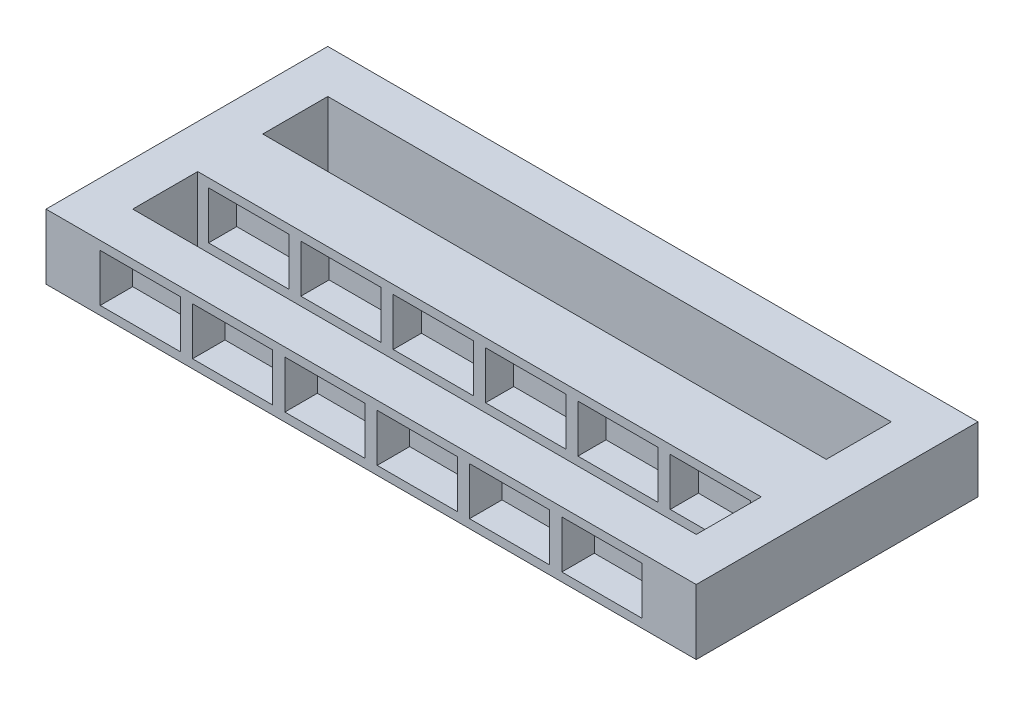
SolidWorks part; units mm, degrees
ref_plane "Front Plane" through (0, 0, 0) normal (0, 0, 1) x (1, 0, 0)
ref_plane "Top Plane" through (0, 0, 0) normal (0, 1, 0) x (1, 0, 0)
ref_plane "Right Plane" through (0, 0, 0) normal (1, 0, 0) x (0, 0, -1)
other "Configuration Table"
sketch "Sketch1" plane through (0, 0, 0) normal (0, 1, 0) x (1, 0, 0)
  line L1 (-1500, 650) -> (1500, 650)
  line L2 (-1500, 650) -> (-1500, -650)
  line L3 (-1500, -650) -> (1500, -650)
  line L4 (1500, 650) -> (1500, -650)
  line L5 (-1500, 650) -> (1500, -650) construction
  line L6 (-1500, -650) -> (1500, 650) construction
  line L7 (-1300, 450) -> (1300, 450)
  line L8 (-1300, 450) -> (-1300, 150)
  line L9 (-1300, 150) -> (1300, 150)
  line L10 (1300, 450) -> (1300, 150)
  line L11 (-1300, -150) -> (1300, -150)
  line L12 (-1300, -150) -> (-1300, -450)
  line L13 (-1300, -450) -> (1300, -450)
  line L14 (1300, -150) -> (1300, -450)
  point P0 (0, 0)
  dimension "D1" = 1300
  dimension "D2" = 3000
  dimension "D3" = 200
  dimension "D4" = 200
  dimension "D5" = 200
  dimension "D6" = 200
  dimension "D7" = 200
  dimension "D8" = 200
  dimension "D9" = 500
  dimension "D10" = 300
extrude "Boss-Extrude1" add sketch "Sketch1" along normal blind 300
sketch "Sketch2" plane through (0, 0, 650) normal (0, 0, 1) x (1, 0, 0)
  line L0 (-1500, 300) -> (-1500, 0) construction
  line L1 (-1250, 260) -> (-880, 260)
  line L2 (-1250, 260) -> (-1250, 40)
  line L3 (-1250, 40) -> (-880, 40)
  line L4 (1250, 260) -> (1250, 40)
  line L5 (1500, 300) -> (1500, 0) construction
  line L6 (-1500, 0) -> (1500, 0) construction
  line L7 (-1500, 300) -> (1500, 300) construction
  line L8 (-880, 260) -> (-880, 40)
  line L9 (-824, 260) -> (-824, 40)
  line L10 (-454, 260) -> (-454, 40)
  line L11 (-398, 260) -> (-398, 40)
  line L12 (-28, 260) -> (-28, 40)
  line L13 (28, 260) -> (28, 40)
  line L14 (398, 260) -> (398, 40)
  line L15 (454, 260) -> (454, 40)
  line L16 (824, 260) -> (824, 40)
  line L17 (880, 260) -> (880, 40)
  line L18 (-824, 260) -> (-454, 260)
  line L19 (-824, 40) -> (-454, 40)
  line L20 (-398, 260) -> (-28, 260)
  line L21 (-398, 40) -> (-28, 40)
  line L22 (28, 260) -> (398, 260)
  line L23 (28, 40) -> (398, 40)
  line L24 (454, 260) -> (824, 260)
  line L25 (454, 40) -> (824, 40)
  line L26 (880, 260) -> (1250, 260)
  line L27 (880, 40) -> (1250, 40)
  dimension "D1" = 250
  dimension "D2" = 250
  dimension "D3" = 40
  dimension "D4" = 40
  dimension "D5" = 56
  dimension "D6" = 56
  dimension "D7" = 56
  dimension "D8" = 56
  dimension "D9" = 56
  dimension "D10" = 370
  dimension "D11" = 370
  dimension "D12" = 370
  dimension "D13" = 370
  dimension "D14" = 370
extrude "Cut-Extrude1" cut sketch "Sketch2" against normal blind 150
mirror "Mirror1" about plane through (0, 0, 0) normal (0, 0, 1) of "Cut-Extrude1"
sketch "Sketch3" plane through (0, 0, 150) normal (0, 0, 1) x (1, 0, 0)
  line L1 (-1250, 260) -> (-880, 260)
  line L2 (-1250, 260) -> (-1250, 40)
  line L3 (-1250, 40) -> (-880, 40)
  line L4 (-880, 260) -> (-880, 40)
  line L5 (-824, 260) -> (-454, 260)
  line L6 (-824, 260) -> (-824, 40)
  line L7 (-824, 40) -> (-454, 40)
  line L8 (-454, 260) -> (-454, 40)
  line L9 (-398, 260) -> (-28, 260)
  line L10 (-398, 260) -> (-398, 40)
  line L11 (-398, 40) -> (-28, 40)
  line L12 (-28, 260) -> (-28, 40)
  line L13 (28, 260) -> (398, 260)
  line L14 (28, 260) -> (28, 40)
  line L15 (28, 40) -> (398, 40)
  line L16 (398, 260) -> (398, 40)
  line L17 (454, 260) -> (824, 260)
  line L18 (454, 260) -> (454, 40)
  line L19 (454, 40) -> (824, 40)
  line L20 (824, 260) -> (824, 40)
  line L21 (880, 260) -> (1250, 260)
  line L22 (880, 260) -> (880, 40)
  line L23 (880, 40) -> (1250, 40)
  line L24 (1250, 260) -> (1250, 40)
extrude "Cut-Extrude2" cut sketch "Sketch3" against normal blind 130
mirror "Mirror2" about plane through (0, 0, 0) normal (0, 0, 1) of "Cut-Extrude2"
